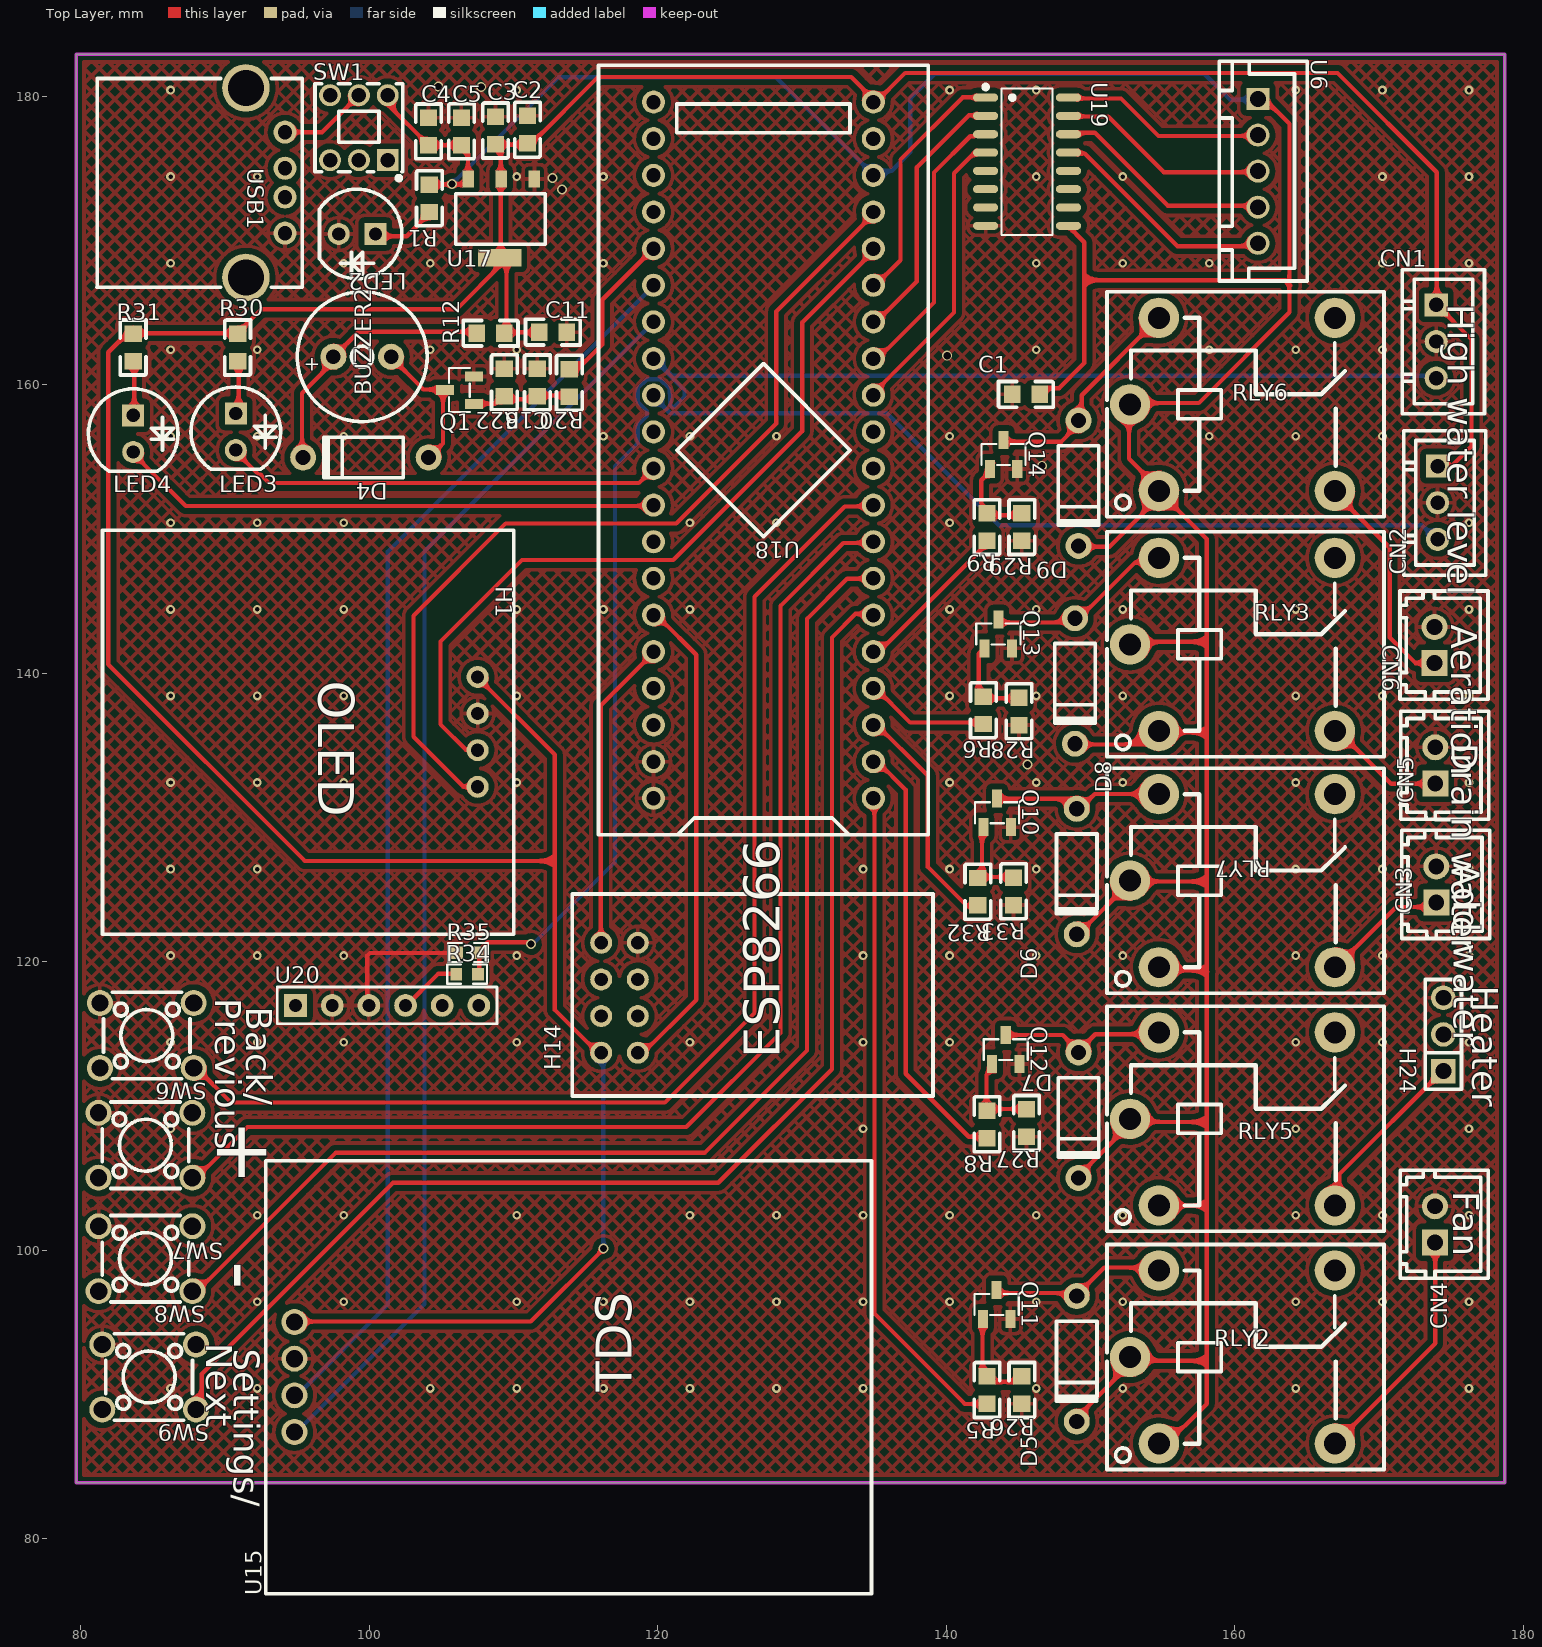
[diagram p0: Top Layer view]
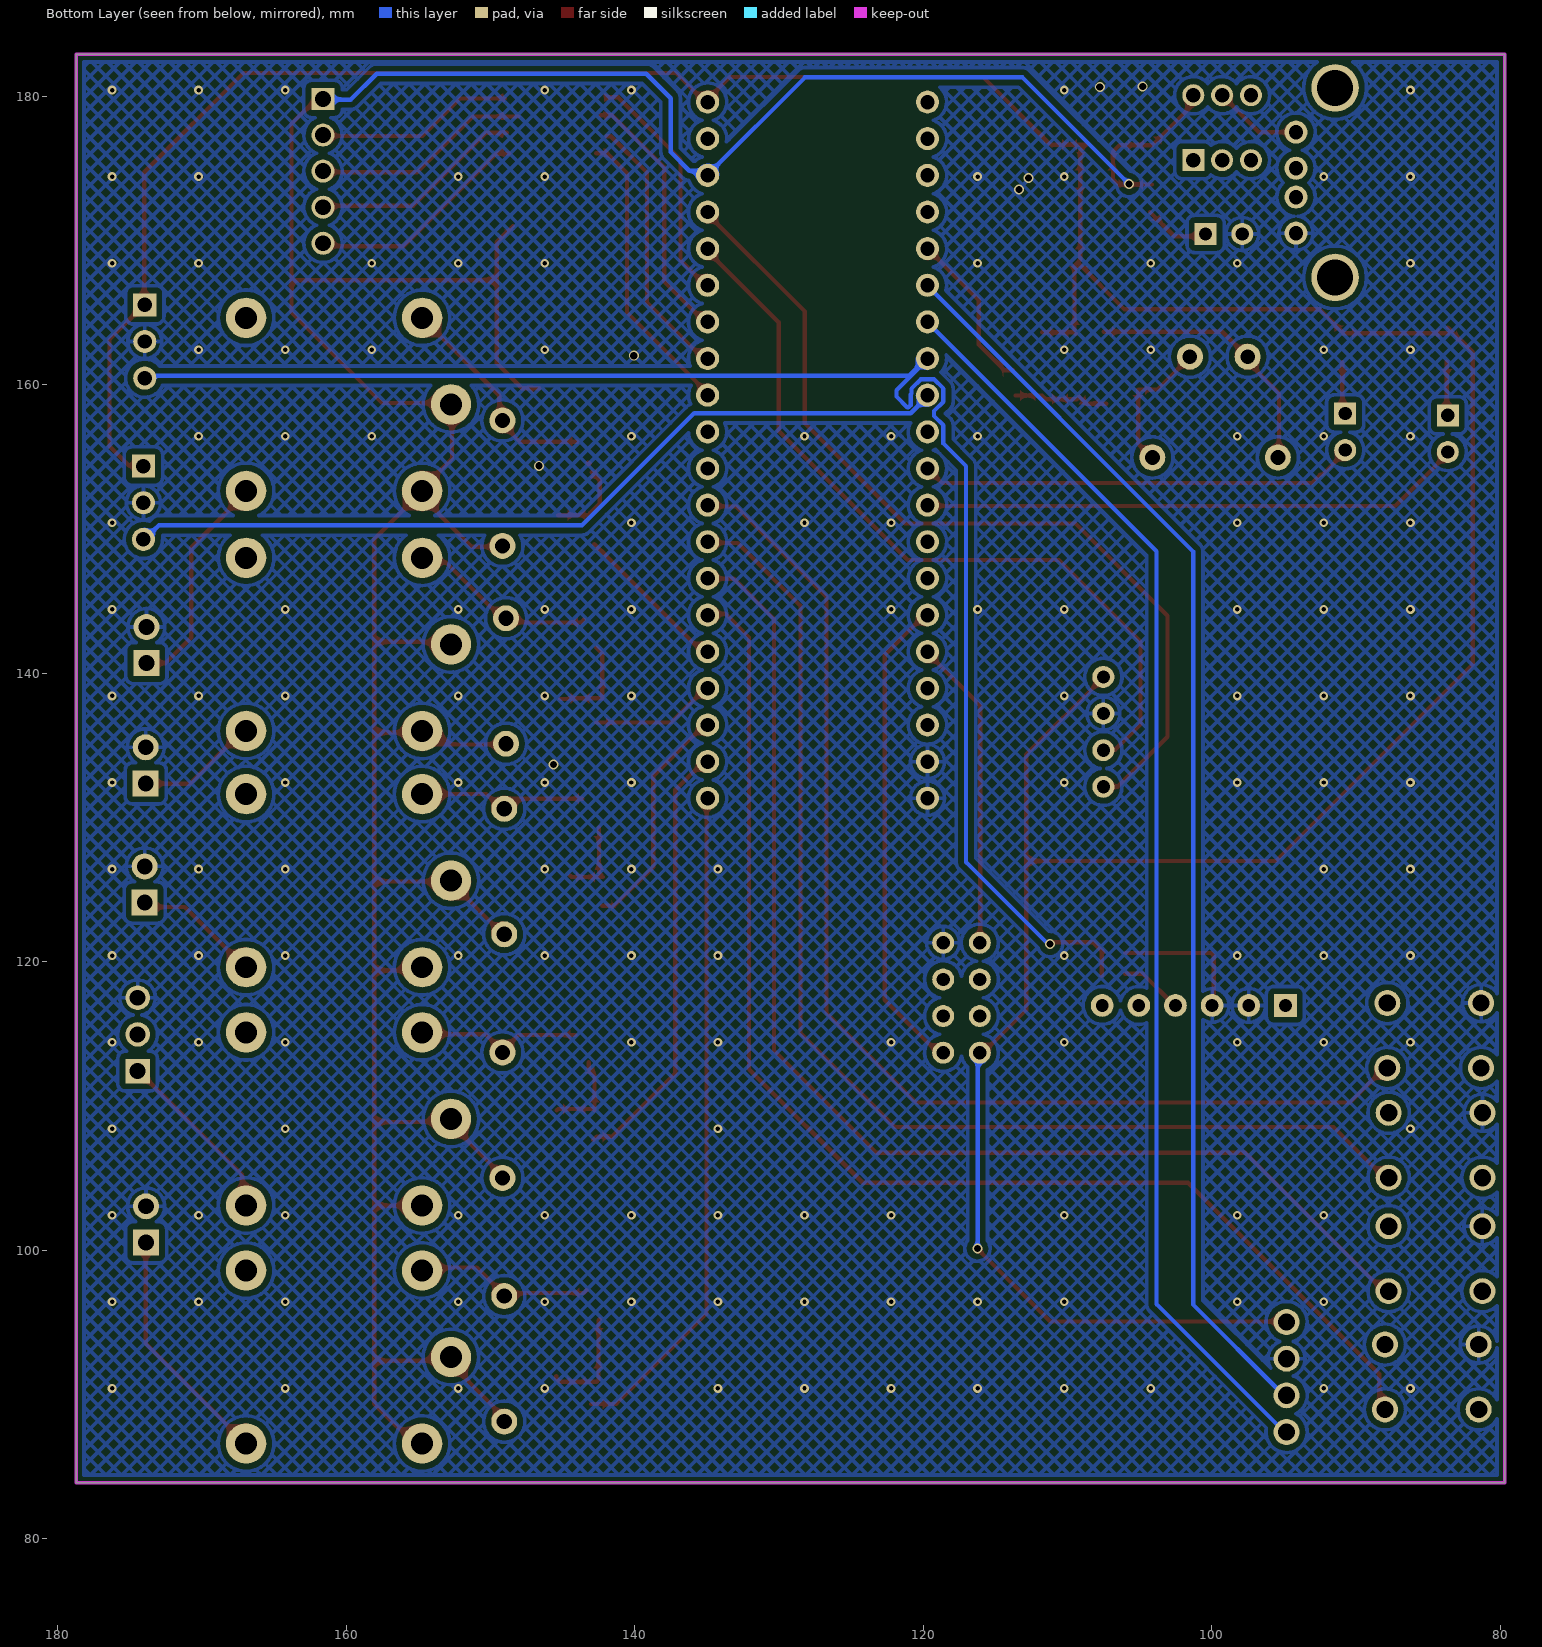
[diagram p1: Bottom Layer view, seen from below]
# Altium PCB MISC62619.pcbdoc
Units mm, origin at the board's own origin, x right, y up, seen from the top; angles counter-clockwise.
Board outline 99 x 99 mm, 2 copper layers (Top Layer, Bottom Layer), stack 1.58 mm thick; 67 components, 55 nets, 245 pads, 159 vias.

## Layer stack, top to bottom
Top Solder Mask Layer: solder mask 0.01, Dk 3.3
Top Layer: signal copper 0.035
Dielectric1: surface 1.51, FR4, Dk 4.5
Bottom Layer: signal copper 0.035
Bottom Solder Mask Layer: solder mask 0.01, Dk 3.3

## Board outline
79.696,182.894 79.696,83.894 178.696,83.894 178.696,182.894

## Design rules (kind name [scope] priority, off if disabled: settings)
BoardOutlineClearance copperThickness2oz_1 [All] p2 off: genericclearance=0.203 ignorepadtopadclearanceinfootprint=FALSE except(0: Arc-SplitContinuation Track-SplitContinuation SMDPad-SplitContinuation THPad-SplitContinuation Via-SplitContinuation Fill-SplitContinuation Region-SplitContinuation Poly-SplitContinuation Text-SplitContinuation Hole-SplitContinuation; 0.152: SMDPad-CutoutEdge THPad-CutoutEdge Via-CutoutEdge Fill-CutoutEdge Region-CutoutEdge Text-CutoutEdge Hole-CutoutEdge; 0.254: Poly-OutlineEdge Poly-CutoutEdge; 0.3: Arc-OutlineEdge Track-OutlineEdge SMDPad-OutlineEdge THPad-OutlineEdge Via-OutlineEdge Fill-OutlineEdge Region-OutlineEdge Text-OutlineEdge Hole-OutlineEdge Arc-CutoutEdge Track-CutoutEdge)
BoardOutlineClearance Plane_innerPlane_1 [All] p4 off: genericclearance=0.102 ignorepadtopadclearanceinfootprint=FALSE except(0: Arc-SplitContinuation Track-SplitContinuation SMDPad-SplitContinuation THPad-SplitContinuation Via-SplitContinuation Fill-SplitContinuation Region-SplitContinuation Poly-SplitContinuation Text-SplitContinuation Hole-SplitContinuation; 0.152: SMDPad-CutoutEdge THPad-CutoutEdge Via-CutoutEdge Fill-CutoutEdge Region-CutoutEdge Text-CutoutEdge Hole-CutoutEdge; 0.254: Poly-OutlineEdge Poly-CutoutEdge; 0.3: Arc-OutlineEdge Track-OutlineEdge SMDPad-OutlineEdge THPad-OutlineEdge Via-OutlineEdge Fill-OutlineEdge Region-OutlineEdge Text-OutlineEdge Hole-OutlineEdge Arc-CutoutEdge Track-CutoutEdge)
BoardOutlineClearance Copper_copperRegion_1 [All] p6 off: genericclearance=0.102 ignorepadtopadclearanceinfootprint=FALSE except(0: Arc-SplitContinuation Track-SplitContinuation SMDPad-SplitContinuation THPad-SplitContinuation Via-SplitContinuation Fill-SplitContinuation Region-SplitContinuation Poly-SplitContinuation Text-SplitContinuation Hole-SplitContinuation; 0.152: SMDPad-CutoutEdge THPad-CutoutEdge Via-CutoutEdge Fill-CutoutEdge Region-CutoutEdge Text-CutoutEdge Hole-CutoutEdge; 0.254: Poly-OutlineEdge Poly-CutoutEdge; 0.3: Arc-OutlineEdge Track-OutlineEdge SMDPad-OutlineEdge THPad-OutlineEdge Via-OutlineEdge Fill-OutlineEdge Region-OutlineEdge Text-OutlineEdge Hole-OutlineEdge Arc-CutoutEdge Track-CutoutEdge)
BoardOutlineClearance Copper_copperRegion1_1 [All] p8 off: genericclearance=0.102 ignorepadtopadclearanceinfootprint=FALSE except(0: Arc-SplitContinuation Track-SplitContinuation SMDPad-SplitContinuation THPad-SplitContinuation Via-SplitContinuation Fill-SplitContinuation Region-SplitContinuation Poly-SplitContinuation Text-SplitContinuation Hole-SplitContinuation; 0.152: SMDPad-CutoutEdge THPad-CutoutEdge Via-CutoutEdge Fill-CutoutEdge Region-CutoutEdge Text-CutoutEdge Hole-CutoutEdge; 0.3: Arc-OutlineEdge Track-OutlineEdge SMDPad-OutlineEdge THPad-OutlineEdge Via-OutlineEdge Fill-OutlineEdge Region-OutlineEdge Text-OutlineEdge Hole-OutlineEdge Arc-CutoutEdge Track-CutoutEdge; 0.4: Poly-OutlineEdge Poly-CutoutEdge)
BoardOutlineClearance copperThickness1oz_1 [All] p10: genericclearance=0.102 ignorepadtopadclearanceinfootprint=FALSE except(0: Arc-SplitContinuation Track-SplitContinuation SMDPad-SplitContinuation THPad-SplitContinuation Via-SplitContinuation Fill-SplitContinuation Region-SplitContinuation Poly-SplitContinuation Text-SplitContinuation Hole-SplitContinuation; 0.152: SMDPad-CutoutEdge THPad-CutoutEdge Via-CutoutEdge Fill-CutoutEdge Region-CutoutEdge Text-CutoutEdge Hole-CutoutEdge; 0.254: Poly-OutlineEdge Poly-CutoutEdge; 0.3: Arc-OutlineEdge Track-OutlineEdge SMDPad-OutlineEdge THPad-OutlineEdge Via-OutlineEdge Fill-OutlineEdge Region-OutlineEdge Text-OutlineEdge Hole-OutlineEdge Arc-CutoutEdge Track-CutoutEdge)
Clearance copperThickness2oz [All] p1 off: gap=0.203 ignorepadtopadclearanceinfootprint=FALSE except(0.152: SMDPad-Track SMDPad-SMDPad THPad-Track SMDPad-THPad THPad-THPad Track-Via SMDPad-Via THPad-Via Via-Via Fill-Track Region-Track Fill-SMDPad Region-SMDPad Fill-THPad Region-THPad Fill-Via Region-Via Fill-Fill Fill-Region Region-Region Arc-Track Arc-SMDPad Arc-THPad Arc-Via Fill-Arc Region-Arc Arc-Arc Text-Track SMDPad-Text Text-THPad Text-Via Fill-Text Region-Text Arc-Text Text-Text Hole-Track Hole-SMDPad Hole-THPad Hole-Via Fill-Hole Region-Hole Hole-Arc Hole-Text; 0.254: Poly-Track Poly-SMDPad Poly-THPad Poly-Via Poly-Fill Poly-Region Poly-Poly Poly-Arc Poly-Text Poly-Hole)
Clearance Plane_innerPlane [All] p3 off: gap=0.102 ignorepadtopadclearanceinfootprint=FALSE except(0.152: SMDPad-Track SMDPad-SMDPad THPad-Track SMDPad-THPad THPad-THPad Track-Via SMDPad-Via THPad-Via Via-Via Fill-Track Region-Track Fill-SMDPad Region-SMDPad Fill-THPad Region-THPad Fill-Via Region-Via Fill-Fill Fill-Region Region-Region Arc-Track Arc-SMDPad Arc-THPad Arc-Via Fill-Arc Region-Arc Arc-Arc Text-Track SMDPad-Text Text-THPad Text-Via Fill-Text Region-Text Arc-Text Text-Text Hole-Track Hole-SMDPad Hole-THPad Hole-Via Fill-Hole Region-Hole Hole-Arc Hole-Text; 0.254: Poly-Track Poly-SMDPad Poly-THPad Poly-Via Poly-Fill Poly-Region Poly-Poly Poly-Arc Poly-Text Poly-Hole)
Clearance Copper_copperRegion [All] p5 off: gap=0.102 ignorepadtopadclearanceinfootprint=FALSE except(0.152: SMDPad-Track SMDPad-SMDPad THPad-Track SMDPad-THPad THPad-THPad Track-Via SMDPad-Via THPad-Via Via-Via Fill-Track Region-Track Fill-SMDPad Region-SMDPad Fill-THPad Region-THPad Fill-Via Region-Via Fill-Fill Fill-Region Region-Region Arc-Track Arc-SMDPad Arc-THPad Arc-Via Fill-Arc Region-Arc Arc-Arc Text-Track SMDPad-Text Text-THPad Text-Via Fill-Text Region-Text Arc-Text Text-Text Hole-Track Hole-SMDPad Hole-THPad Hole-Via Fill-Hole Region-Hole Hole-Arc Hole-Text; 0.254: Poly-Track Poly-SMDPad Poly-THPad Poly-Via Poly-Fill Poly-Region Poly-Poly Poly-Arc Poly-Text Poly-Hole)
Clearance Copper_copperRegion1 [All] p7 off: gap=0.102 ignorepadtopadclearanceinfootprint=FALSE except(0.152: SMDPad-Track SMDPad-SMDPad THPad-Track SMDPad-THPad THPad-THPad Track-Via SMDPad-Via THPad-Via Via-Via Fill-Track Region-Track Fill-SMDPad Region-SMDPad Fill-THPad Region-THPad Fill-Via Region-Via Fill-Fill Fill-Region Region-Region Arc-Track Arc-SMDPad Arc-THPad Arc-Via Fill-Arc Region-Arc Arc-Arc Text-Track SMDPad-Text Text-THPad Text-Via Fill-Text Region-Text Arc-Text Text-Text Hole-Track Hole-SMDPad Hole-THPad Hole-Via Fill-Hole Region-Hole Hole-Arc Hole-Text; 0.4: Poly-Track Poly-SMDPad Poly-THPad Poly-Via Poly-Fill Poly-Region Poly-Poly Poly-Arc Poly-Text Poly-Hole)
Clearance copperThickness1oz [All] p9: gap=0.102 ignorepadtopadclearanceinfootprint=FALSE except(0.152: SMDPad-Track SMDPad-SMDPad THPad-Track SMDPad-THPad THPad-THPad Track-Via SMDPad-Via THPad-Via Via-Via Fill-Track Region-Track Fill-SMDPad Region-SMDPad Fill-THPad Region-THPad Fill-Via Region-Via Fill-Fill Fill-Region Region-Region Arc-Track Arc-SMDPad Arc-THPad Arc-Via Fill-Arc Region-Arc Arc-Arc Text-Track SMDPad-Text Text-THPad Text-Via Fill-Text Region-Text Arc-Text Text-Text Hole-Track Hole-SMDPad Hole-THPad Hole-Via Fill-Hole Region-Hole Hole-Arc Hole-Text; 0.254: Poly-Track Poly-SMDPad Poly-THPad Poly-Via Poly-Fill Poly-Region Poly-Poly Poly-Arc Poly-Text Poly-Hole)
DiffPairsRouting differentialPair [All] p1: maxlimit=0.152 minlimit=0.152 mostfreqgap=0.152 toplayer_minwidth=0.127 toplayer_prefwidth=0.254 toplayer_maxwidth=2.54 toplayer_mingap=0.152 toplayer_prefgap=0.152 toplayer_maxgap=0.152 bottomlayer_minwidth=0.127 bottomlayer_prefwidth=0.254 bottomlayer_maxwidth=2.54 bottomlayer_mingap=0.152 bottomlayer_prefgap=0.152 bottomlayer_maxgap=0.152 maxuncoupledlength=0.254
HoleToHoleClearance otherClearance [All] p1: gap=0.3 allowstackedmicrovias=TRUE
Length netLength [All] p1: minlimit=0 maxlimit=0
PasteMaskExpansion pasteMaskExpansion [All] p1: expansion=0
PlaneConnect innerPlane [All] p1: planeconnectstyle=Relief reliefexpansion=0.508 reliefentries=4 reliefconductorwidth=0.254 reliefairgap=0.254
PolygonConnect copperRegion1 [All] p1 off: connectstyle=Relief reliefconductorwidth=0.254 reliefentries=4 polygonreliefangle="90 Angle" airgapwidth=0.254 via.connectstyle=Relief via.reliefconductorwidth=0.254 via.reliefentries=4 via.polygonreliefangle="90 Angle" via.airgapwidth=0.254
PolygonConnect copperRegion [All] p2: connectstyle=Relief reliefconductorwidth=0.254 reliefentries=4 polygonreliefangle="90 Angle" airgapwidth=0.254 via.connectstyle=Relief via.reliefconductorwidth=0.254 via.reliefentries=4 via.polygonreliefangle="90 Angle" via.airgapwidth=0.254
RoutingVias viaSize [All] p1: holewidth=0.305 width=0.61 viastyle="Through Hole" minholewidth=0.3 minwidth=0.5 maxholewidth=6.3 maxwidth=10
SolderMaskExpansion solderMaskExpansion [IsVia] p1: expansion=-25.4 istentingtop=TRUE
SolderMaskExpansion solderMaskExpansion [All] p2: expansion=0.051 istentingtop=FALSE
Width copperThickness2oz_2 [All] p1 off: maxlimit=2.54 minlimit=0.203 preferedwidth=0.254
Width copperThickness1oz_2 [All] p2: maxlimit=2.54 minlimit=0.127 preferedwidth=0.254

## Components (designator, comment, footprint, x,y, rotation, side; value= is the part's Value field where it differs from the comment)
BUZZER2 "2.7kHz" BUZ-TH_BD9.0-P4.00-D0.6-FD 99.508,161.939 r0 top
C1 "100nF" c0805 145.515,159.327 r0 top
C2 "0.1u" c0805 110.961,177.682 r270 top
C3 "10u" c0805 108.746,177.621 r270 top
C4 "10u" c0805 104.103,177.555 r270 top
C5 "0.1u" c0805 106.384,177.56 r270 top
C11 "104/0603" c0805 112.726,163.637 r180 top
C16 "104/0603" c0805 111.644,160.149 r270 top
CN1 "ZX-XH2.54-3PZZ" CONN-TH_3P-P2.54_2501S-3P 173.956,162.995 r270 top
CN2 "ZX-XH2.54-3PZZ" CONN-TH_3P-P2.54_2501S-3P 174.05,151.817 r270 top
CN3 "ZX-XH2.54-2PZZ" CONN-TH_2P-P2.50_HX25003-2A 173.961,125.357 r90 top
CN4 "ZX-XH2.54-2PZZ" CONN-TH_2P-P2.50_HX25003-2A 173.867,101.798 r90 top
CN5 "ZX-XH2.54-2PZZ" CONN-TH_2P-P2.50_HX25003-2A 173.891,133.615 r90 top
CN6 "ZX-XH2.54-2PZZ" CONN-TH_2P-P2.50_HX25003-2A 173.843,141.95 r90 top
D4 "1N4007" DO-41_BD2.4-L4.7-P8.70-D0.8-RD 99.762,154.954 r0 top
D5 "1N4007" DO-41_BD2.4-L4.7-P8.70-D0.8-RD 149.038,92.47 r90 top
D6 "1N4007" DO-41_BD2.4-L4.7-P8.70-D0.8-RD 149.038,126.252 r90 top
D7 "1N4007" DO-41_BD2.4-L4.7-P8.70-D0.8-RD 149.165,109.361 r90 top
D8 "1N4007" DO-41_BD2.4-L4.7-P8.70-D0.8-RD 148.911,139.46 r90 top
D9 "1N4007" DO-41_BD2.4-L4.7-P8.70-D0.8-RD 149.165,153.176 r90 top
H1 "OLED" oled 107.509,135.904 r270 top
H14 "PZ254V-12-8P" esp8266 116.073,117.691 r90 top
H24 "Heater" HDR-TH_3P-P2.54-V-M 174.454,114.961 r90 top
LED2 "L-7113SGC" LED-TH_BD5.9-P2.54-FD 99.15,170.448 r180 top
LED3 "L-7113SGC" LED-TH_BD5.9-P2.54-FD 90.745,156.732 r270 top
LED4 "L-7113SGC" LED-TH_BD5.9-P2.54-FD 83.633,156.605 r270 top
Q1 "SS8050/SOT23-3" SOT-23-3_L2.9-W1.3-P1.90-LS2.4-BR 106.242,159.623 r0 top
Q10 "SS8050/SOT23-3" SOT-23-3_L2.9-W1.3-P1.90-LS2.4-BR 143.517,130.324 r270 top
Q11 "SS8050/SOT23-3" SOT-23-3_L2.9-W1.3-P1.90-LS2.4-BR 143.486,96.231 r270 top
Q12 "SS8050/SOT23-3" SOT-23-3_L2.9-W1.3-P1.90-LS2.4-BR 144.116,113.905 r270 top
Q13 "SS8050/SOT23-3" SOT-23-3_L2.9-W1.3-P1.90-LS2.4-BR 143.603,142.722 r270 top
Q14 "SS8050/SOT23-3" SOT-23-3_L2.9-W1.3-P1.90-LS2.4-BR 143.965,155.161 r270 top
R1 "" c0805 104.164,172.922 r270 top
R5 "" c0805 142.815,90.311 r90 top
R6 "" c0805 142.561,137.428 r90 top
R8 "" c0805 142.815,108.726 r90 top
R9 "" c0805 142.815,150.128 r90 top
R12 "220" c0805 108.406,163.565 r180 top
R20 "1K/0603" c0805 113.862,160.126 r270 top
R22 "10K/0603" c0805 109.361,160.162 r270 top
R26 "10K/0603" c0805 145.228,90.311 r90 top
R27 "10K/0603" c0805 145.55,108.827 r90 top
R28 "10K/0603" c0805 145.04,137.357 r90 top
R29 "10K/0603" c0805 145.228,150.128 r90 top
R30 "" c0805 90.872,162.574 r90 top
R31 "" c0805 83.633,162.574 r90 top
R32 "" c0805 142.18,124.855 r90 top
R33 "10K/0603" c0805 144.654,124.879 r90 top
R34 "2.2K" R0603 106.782,119.138 r0 top
R35 "3.3K" R0603 106.834,120.636 r0 top
RLY2 "SRD-05VDC-SL-C" RELAY-TH_SRD-XXVDC-XL-C 159.833,92.597 r0 top
RLY3 "SRD-05VDC-SL-C" RELAY-TH_SRD-XXVDC-XL-C 159.833,142 r0 top
RLY5 "SRD-05VDC-SL-C" RELAY-TH_SRD-XXVDC-XL-C 159.833,109.107 r0 top
RLY6 "SRD-05VDC-SL-C" RELAY-TH_SRD-XXVDC-XL-C 159.833,158.637 r0 top
RLY7 "SRD-05VDC-SL-C" RELAY-TH_SRD-XXVDC-XL-C 159.833,125.617 r0 top
SW1 "5.8 ZSGT" SW-TH_5.8ZSGT 99.277,177.814 r0 top
SW6 "TS665CJ" SW-TH_4P-L6.0-W6.0-P4.50-LS6.5 84.575,114.883 r180 top
SW7 "TS665CJ" SW-TH_4P-L6.0-W6.0-P4.50-LS6.5 84.48,107.28 r180 top
SW8 "TS665CJ" SW-TH_4P-L6.0-W6.0-P4.50-LS6.5 84.484,99.414 r180 top
SW9 "TS665CJ" SW-TH_4P-L6.0-W6.0-P4.50-LS6.5 84.738,91.217 r180 top
U6 "ZX-XH2.54-5PZZ" CONN-TH_5P-P2.50_ZX-XH2.54-5PZZ 161.602,174.802 r270 top
U15 "" TDS模块 94.809,91.2 r90 top
U17 "AMS1117-3.3" sot-223 111.446,174.258 r270 top
U18 "LCKFB-DKX-STM32F103C8T6" CONN-TH_L53.3-W22.9_STM32F103C8T6-CARD 127.321,155.462 r90 top
U19 "ULN2003A" SOP-16_L10.0-W3.9-P1.27-LS6.0-BL 145.594,175.457 r270 top
U20 "" HDR-M-2.54_1X6 101.239,116.969 r0 top
USB1 "USB-231-ARY" USB-A-TH_USB-231-ARY 92.8,174.004 r270 top

## Footprints (in the part's own frame and the unit in brackets; to place one, negate y for a bottom-side part, rotate by r counter-clockwise, add the part's x,y. Pads: shape width x height; smd on the part's side, far side on the other; paste and mask are expansions set on the pad)
BUZ-TH_BD9.0-P4.00-D0.6-FD [mm]
  round 1.8 hole 1: 1(-2,0) 2(2,0)
  silkscreen extent -4.5,-4.5 4.5,4.5
c0805 [mm]
  rect 1.14x1.2 smd: 1(-0.95,0) 2(0.95,0)
  silkscreen extent -1.91,-0.89 1.91,0.89
CONN-TH_2P-P2.50_HX25003-2A [mm]
  rect 1.8x1.8 hole 1.1 paste+0 mask+0.05: 1(-1.25,0)
  round 1.8 hole 1.1 paste+0 mask+0.05: 2(1.25,0)
  silkscreen extent -3.75,-3.7 3.75,2.41
CONN-TH_3P-P2.54_2501S-3P [mm]
  rect 1.6x1.6 hole 1: 1(-2.54,0)
  round 1.6 hole 1: 2(0,0) 3(2.54,0)
  silkscreen extent -4.98,-2.35 5.02,3.35
CONN-TH_5P-P2.50_ZX-XH2.54-5PZZ [mm]
  rect 1.524x1.6 hole 1.1: 1(-5,0)
  round 1.6 hole 1.1: 2(-2.5,0) 3(0,0) 4(2.5,0) 5(5,0)
  silkscreen extent -7.62,-2.68 7.62,3.42
CONN-TH_L53.3-W22.9_STM32F103C8T6-CARD [mm]
  round 1.6 hole 1: 1(-24.13,-7.62) 2(-21.59,-7.62) 3(-19.05,-7.62) 4(-16.51,-7.62) 5(-13.97,-7.62) 6(-11.43,-7.62) 7(-8.89,-7.62) 8(-6.35,-7.62) 9(-3.81,-7.62) 10(-1.27,-7.62) 11(1.27,-7.62) 12(3.81,-7.62) 13(6.35,-7.62) 14(8.89,-7.62) 15(11.43,-7.62) 16(13.97,-7.62) 17(16.51,-7.62) 18(19.05,-7.62) 19(21.59,-7.62) 20(24.13,-7.62) 21(24.13,7.62) 22(21.59,7.62) 23(19.05,7.62) 24(16.51,7.62) 25(13.97,7.62) 26(11.43,7.62) 27(8.89,7.62) 28(6.35,7.62) 29(3.81,7.62) 30(1.27,7.62) 31(-1.27,7.62) 32(-3.81,7.62) 33(-6.35,7.62) 34(-8.89,7.62) 35(-11.43,7.62) 36(-13.97,7.62) 37(-16.51,7.62) 38(-19.05,7.62) 39(-21.59,7.62) 40(-24.13,7.62)
  silkscreen extent -26.67,-11.43 26.67,11.43
DO-41_BD2.4-L4.7-P8.70-D0.8-RD [mm]
  round 1.8 hole 1.05: 1(-4.35,0) 2(4.35,0)
  silkscreen extent -2.92,-1.4 2.6,1.4
esp8266 [mil]
  round 60 hole 36: 1(-157.48,0) 2(-157.48,-100) 3(-57.48,0) 4(-57.48,-100) 5(42.52,0) 6(42.52,-100) 7(142.52,0) 8(142.52,-100)
  silkscreen extent -276,-906 276,79
HDR-M-2.54_1X6 [mil]
  rect 62x62 hole 35: 1(-250,0)
  round 62 hole 35: 2(-150,0) 3(-50,0) 4(50,0) 5(150,0) 6(250,0)
  silkscreen extent -300,-50 300,50
HDR-TH_3P-P2.54-V-M [mm]
  rect 1.7x1.7 hole 1.1: 1(-2.54,0)
  round 1.7 hole 1.1: 2(0,0) 3(2.54,0)
  silkscreen extent -3.81,-1.25 3.81,1.25
LED-TH_BD5.9-P2.54-FD [mil]
  rect 60x60 hole 36: 1(-50,0)
  round 60 hole 36: 2(50,0)
  silkscreen extent -122,-122 102,122
oled [mil]
  round 60 hole 36: 1(148.82,0) 2(48.82,0) 3(-51.18,0) 4(-151.18,0)
  silkscreen extent -551,-1024 551,98
R0603 [mm]
  rect 0.806x0.864 smd paste-100 mask+0.051: 1(-0.753,0) 2(0.753,0)
  silkscreen extent -1.39,-0.66 1.39,0.66
RELAY-TH_SRD-XXVDC-XL-C [mil]
  round 110 hole 60: 1(-200.79,-236.22) 2(279.52,-236.2) 3(279.53,236.2) 4(-200.79,236.22) 5(-279.53,0)
  silkscreen extent -342,-307 413,307
SOP-16_L10.0-W3.9-P1.27-LS6.0-BL [mm]
  oval 0.56x1.745 smd: 1(-4.445,-2.872) 2(-3.175,-2.872) 3(-1.905,-2.872) 4(-0.635,-2.872) 5(0.635,-2.872) 6(1.905,-2.872) 7(3.175,-2.872) 8(4.445,-2.872) 9(4.445,2.872) 10(3.175,2.872) 11(1.905,2.872) 12(0.635,2.872) 13(-0.635,2.872) 14(-1.905,2.872) 15(-3.175,2.872) 16(-4.445,2.872)
  silkscreen extent -5.33,-3.02 5.08,1.77
SOT-23-3_L2.9-W1.3-P1.90-LS2.4-BR [mm]
  rect 1.25x0.7 smd: 1(1,-0.95) 2(1,0.95) 3(-1,0)
  silkscreen extent -0.73,-1.53 0.73,1.53
sot-223 [mm]
  rect 1.2x0.8 smd: 1(0,0) 2(0,-2.3) 3(0,-4.6)
  rect 1.2x3 smd: 4(5.461,-2.413)
  silkscreen extent 1.02,-5.46 4.52,0.74
SW-TH_4P-L6.0-W6.0-P4.50-LS6.5 [mm]
  round 1.8 hole 1.2: 1(-3.25,2.25) 2(3.25,2.25) 3(-3.25,-2.25) 4(3.25,-2.25)
  silkscreen extent -3,-3 3,3
SW-TH_5.8ZSGT [mm]
  rect 1.524x1.524 hole 1: 1(2,-2.25)
  round 1.524 hole 1: 2(0,-2.25) 3(-2,-2.25) 4(2,2.25) 5(0,2.25) 6(-2,2.25)
  silkscreen extent -3.05,-3.64 3.05,3.05
TDS模块 [mm]
  round 1.8 hole 1.2: 1(-3.8,0) 2(-1.26,0) 3(1.28,0) 4(3.82,0)
  silkscreen extent -15,-40 15,2
USB-A-TH_USB-231-ARY [mm]
  round 1.6 hole 1: 1(-3.5,1.355) 2(-1,1.355) 3(1,1.355) 4(3.5,1.355)
  round 3.3 hole 2.5: 5(-6.57,-1.355) 6(6.57,-1.355)
  silkscreen extent -7.23,-11.68 7.24,2.54

## Via types
v1: diameter 0.61, hole 0.305, Top Layer to Bottom Layer, 149 vias
v2: diameter 0.7, hole 0.5, Top Layer to Bottom Layer, 10 vias

## Nets (pads, with @x,y where several pads share a name; then routed paths per layer and width w, separated by ;. In a path a pad name is that pad's centre, name@x,y a point inside that pad or via, vN(x,y) a via of type N, cw(c..) or ccw(c..) an arc to the next point about the centre after c; other vN are vias at no path point)
3.3V: C2.2 C3.2 C11.2 CN1.1 CN2.1 H1.4 H14.1 R12.1 R30.2 R31.2 U15.4 U17.2 U17.4 U18.20 | length 265.4
  Top Layer w0.3: R31.2@83.574,163.591 83.596,163.569 R30.2@90.895,163.569 ; R31.2@83.626,163.968 81.905,162.247 81.905,140.613 95.532,126.986 112.846,126.986 ; R30.2@90.842,163.571 92.493,165.222 106.038,165.222 U17.4@109.275,168.459 ; U15.4@94.801,95.059 111.192,95.059 v2@116.295,100.162 ; H1.4@107.612,139.592 112.863,134.342 112.863,116.659 H14.1@115.995,113.527 ; U17.4@109.14,168.672 109.111,168.701 109.111,176.219 108.689,176.642 111.005,176.642 C2.2@111.064,176.584 ; U17.4@109.189,168.564 109.514,168.24 R12.1@109.514,163.769 ; R12.1@109.428,163.536 109.516,163.624 C11.2@111.745,163.624 ; C2.2@111.225,176.691 115.858,181.324 133.407,181.324 U18.20@135.046,179.685 ; U18.20@134.985,179.447 137.139,181.601 167.117,181.601 173.997,174.721 CN1.1@173.997,165.548 ; CN1.1@173.807,165.737 CN1.1@173.997,165.548 ; CN1.1@173.997,165.535 CN1.1@173.997,165.548 ; CN2.1@174.018,154.393 175.072,154.393 176.406,155.728 176.406,163.138 CN1.1@173.997,165.548
  Bottom Layer w0.3: H14.1@116.224,113.697 116.224,100.132 v2(116.235,100.12)
5V: C1.2 C4.2 C5.2 D5.1 D6.1 D7.1 D8.1 D9.1 R1.1 RLY2.1 RLY2.5 RLY3.1 RLY3.5 RLY5.1 RLY5.5 RLY6.1 RLY6.5 RLY7.1 RLY7.5 SW1.4 U6.1 U17.3 U18.18 U19.9 | length 273.1
  Top Layer w0.3: SW1.4 101.277,179.431 C4.2 106.379,176.605 C5.2 106.846,176.148 U17.3 106.46,173.872 R1.1 ; C1.2@146.591,159.764 147.826,159.764 149.565,161.502 149.565,167.244 ; U19.9@148.427,171 149.554,169.873 ; D6.1@148.84,122.055 149.292,122.055 RLY7.5@152.711,125.473 ; D5.1@149.022,88.387 RLY2.5@152.971,92.337 ; D7.1@149.128,105.128 RLY5.5@152.89,108.89 ; D8.1@149.145,135.057 RLY3.1@153.931,135.057 ; D9.1@149.178,148.76 151.308,148.76 154.882,152.333 RLY6.1@154.882,152.47 ; 149.565,169.873 149.565,167.244 ; RLY6.5@152.664,158.731 157.503,158.731 163.789,165.018 163.789,166.942 ; RLY6.5@152.665,158.638 152.665,154.868 RLY6.1@154.96,152.574 ; RLY3.5@152.7,142.178 158.013,142.178 158.041,142.149 ; RLY2.5@152.705,92.337 RLY2.5@152.971,92.337 ; RLY7.5@152.804,125.567 158.018,125.567 ; RLY5.5@152.921,108.921 RLY5.5@152.89,108.89 ; RLY6.1@154.751,152.601 RLY6.1@154.882,152.47 ; RLY3.1@154.753,135.885 158.041,135.885 158.052,135.895 ; RLY5.1@154.8,103.089 157.984,103.089 157.994,103.099 ; RLY7.1@154.81,119.39 158.026,119.39 158.052,119.363 ; RLY2.1@154.953,86.252 158.052,89.352 158.052,108.89 ; 158.044,92.337 RLY2.5@153.096,92.337 ; 158.072,108.9 158.062,108.89 158.052,108.89 ; 158.072,135.916 158.052,135.895 ; 158.104,119.312 158.052,119.363 ; U6.1@161.928,179.944 163.789,178.083 163.789,166.942 ; 163.858,166.873 163.789,166.942 ; 149.565,167.244 163.487,167.244 163.789,166.942 ; RLY5.5@152.89,108.89 158.052,108.89 ; RLY2.5@152.971,92.337 RLY2.5@153.096,92.337 ; RLY2.5@152.971,92.337 152.986,92.352 RLY2.5@153.096,92.337 ; RLY6.1@154.882,152.47 158.052,149.3 158.052,135.895 ; 158.052,108.89 158.052,119.363 ; 158.052,119.363 158.052,135.895
  Bottom Layer w0.3: v2(105.729,173.914) 113.117,181.302 128.201,181.302 U18.18@134.913,174.59 ; U18.18@134.794,174.584 U18.18@134.908,174.469 ; U18.18@134.95,174.531 135.25,174.831 136.207,174.831 137.499,176.124 137.499,179.859 139.196,181.556 157.88,181.556 159.675,179.761 U6.1@161.735,179.761
$1N861: U6.5 U19.13 | length 15.6
  Top Layer w0.3: U19.13@148.694,176.028 149.599,176.028 156.026,169.6 U6.5@161.616,169.6
$1N862: U6.4 U19.14 | length 14.7
  Top Layer w0.3: U19.14@148.872,177.461 150.295,177.461 155.343,172.413 U6.4@161.448,172.413
$1N863: U6.3 U19.15 | length 15.2
  Top Layer w0.3: U19.15@148.066,178.586 151.219,178.586 155.071,174.734 U6.3@161.677,174.734
$1N864: U6.2 U19.16 | length 13.9
  Top Layer w0.3: U19.16@149.003,179.834 149.006,179.837 152.102,179.837 154.704,177.235 161.79,177.235 U6.2@161.794,177.239
$1N1483: D5.2 Q11.3 RLY2.4 | length 12.5
  Top Layer w0.3: Q11.3@143.321,97.236 143.517,97.04 149.179,97.04 150.95,98.81 154.509,98.81 RLY2.4@154.873,98.446
$1N1484: CN4.1 RLY2.2 | length 16.6
  Top Layer w0.3: RLY2.2@167.061,86.716 173.888,93.543 CN4.1@173.888,100.51
$1N1737: D8.2 Q13.3 RLY3.4 | length 13.5
  Top Layer w0.3: Q13.3@143.518,143.714 143.716,143.516 D8.2@148.917,143.516 ; D8.2@149.188,143.516 D8.2@148.917,143.516 ; RLY3.4@154.947,147.678 153.079,147.678 D8.2@148.917,143.516
$1N1738: CN5.1 RLY3.2 | length 8.2
  Top Layer w0.3: RLY3.2@167.271,135.901 170.83,132.342 CN5.1@174.038,132.342
$1N2245: D7.2 Q12.3 RLY5.4 | length 11.5
  Top Layer w0.3: Q12.3@144.102,114.918 148.062,114.918 D7.2@149.165,113.814 ; D7.2@149.184,113.796 D7.2@149.165,113.814 ; RLY5.4@154.685,114.974 150.325,114.974 D7.2@149.165,113.814
$1N2246: H24.1 RLY5.2 | length 12.8
  Top Layer w0.3: RLY5.2@167.224,102.864 167.224,105.251 H24.1@174.553,112.58
$1N2555: D9.2 Q14.3 RLY6.4 | length 15.1
  Top Layer w0.3: Q14.3@143.968,156.055 147.98,156.055 D9.2@149.358,157.432 ; D9.2@149.385,157.305 149.385,159.272 154.47,164.357 RLY6.4@154.485,164.342
$1N2556: CN6.1 RLY6.2 | length 15.6
  Top Layer w0.3: RLY6.2@166.996,152.437 170.736,148.697 170.736,142.48 172.516,140.701 CN6.1@174.061,140.701
$1N5721: LED2.1 R1.2 | length 4.5
  Top Layer w0.3: LED2.1@100.442,170.289 102.599,170.289 R1.2@104.274,171.965
$1N6173: C16.2 Q1.1 R20.2 R22.2 | length 6.7
  Top Layer w0.3: Q1.1@107.309,158.681 108.707,158.681 109.188,159.162 109.363,158.987 111.505,158.987 111.767,159.25 R20.2@113.603,159.25
$1N6175: BUZZER2.2 D4.2 Q1.3 | length 9.9
  Top Layer w0.3: BUZZER2.2@101.342,162.069 103.746,159.665 105.101,159.665 105.101,155.928 D4.2@104.074,154.901
$1N6178: BUZZER2.1 D4.1 R12.2 | length 18.5
  Top Layer w0.3: D4.1@95.332,154.86 95.332,159.406 BUZZER2.1@97.627,161.701 ; BUZZER2.1@97.517,161.919 99.266,163.667 R12.2@107.483,163.667
$1N8726: Q11.1 R5.2 R26.2 | length 7.5
  Top Layer w0.3: Q11.1@142.429,95.211 142.501,95.139 142.501,91.008 142.632,90.876 145.186,90.876 145.432,91.122 R26.2@145.432,91.278
$1N8768: Q12.1 R8.2 R27.2 | length 6
  Top Layer w0.3: R8.2@142.785,109.696 142.785,112.154 143.19,112.56 Q12.1@143.19,113.024 ; R8.2@142.981,109.794 145.309,109.794 R27.2@145.407,109.696
$1N8808: Q13.1 R6.2 R28.2 | length 6.6
  Top Layer w0.3: Q13.1@142.668,141.782 142.236,141.35 142.236,138.255 144.552,138.255 144.596,138.211 R28.2@145.157,138.211
$1N8848: Q14.1 R9.2 R29.2 | length 5.8
  Top Layer w0.3: Q14.1@142.965,153.929 142.415,153.38 142.415,151.773 R9.2@143.069,151.118 ; R9.2@143.069,150.953 145.294,150.953 R29.2@145.304,150.963 ; Q14.1@143.106,154.553 143.173,154.486 143.24,154.553 143.24,154.578 Q14.1@143.228,154.589
$1N8939: LED3.1 R30.1 | length 3.6
  Top Layer w0.3: LED3.1@90.742,158.018 90.939,158.215 R30.1@90.939,161.559
$1N8963: LED4.1 R31.1 | length 3.8
  Top Layer w0.3: LED4.1@83.64,157.821 83.705,157.887 R31.1@83.705,161.602
$1N9376: D6.2 Q10.3 RLY7.4 | length 12
  Top Layer w0.3: Q10.3@143.64,131.302 148.519,131.302 D6.2@149.158,130.663 ; D6.2@149.21,130.556 150.281,131.627 RLY7.4@154.936,131.627
$1N9377: CN3.1 RLY7.2 | length 8.9
  Top Layer w0.3: RLY7.2@166.967,119.582 171.181,123.796 CN3.1@174.155,123.796
$1N9379: Q10.1 R32.2 R33.2 | length 5.6
  Top Layer w0.3: R32.2@142.206,125.877 144.372,125.877 R33.2@144.466,125.971 ; R32.2@142.299,126.017 142.471,126.189 Q10.1@142.471,129.291
$1N14885: SW1.5 USB1.1 | length 6.2
  Top Layer w0.3: USB1.1@94.155,177.504 96.717,177.504 SW1.5
$1N31715: R34.1 U20.4 | length 4.4
  Top Layer w0.3: U20.4@102.558,116.949 104.767,119.158 R34.1@106,119.158
+5V: U20.1
ACC: SW7.1 U18.8 | length 83.1
  Top Layer w0.3: SW7.1@87.597,104.83 87.842,104.83 91.554,108.543 121.976,108.543 128.497,115.064 128.497,144.668 132.857,149.028 134.824,149.028 U18.8@134.977,149.181
ACC_WATER: R32.1 U18.3 | length 16.3
  Top Layer w0.3: U18.3@134.924,136.685 138.717,132.892 138.717,126.571 141.398,123.89 R32.1@142.245,123.89
AIR: R9.1 U18.5 | length 11
  Top Layer w0.3: U18.5@134.819,141.532 135.38,141.532 R9.1@142.791,148.942
BACK: SW6.1 U18.9 | length 82.3
  Top Layer w0.3: SW6.1@87.756,112.475 88.18,112.475 90.413,110.242 120.489,110.242 126.701,116.454 126.701,145.303 132.951,151.553 U18.9@135.093,151.553
BUZZER_CTRL: R20.1 U18.25 | length 11.1
  Top Layer w0.3: R20.1@113.775,161.002 114.368,161.002 116.147,162.782 116.147,165.888 U18.25@119.581,169.322
DEC: SW8.1 U18.7 | length 85.6
  Top Layer w0.3: SW8.1@87.469,96.555 97.664,106.75 123.241,106.75 130.337,113.846 130.337,143.765 133.12,146.548 U18.7@134.857,146.548
DEC_WATER: R6.1 U18.4 | length 8.7
  Top Layer w0.3: U18.4@134.994,139.074 137.488,136.58 R6.1@142.65,136.58
ES8266_TX: H14.7 U18.36 | length 21.6
  Top Layer w0.3: H14.7@116.047,121.343 116.047,137.762 U18.36@119.732,141.447
ESP8266_RX: H14.2 U18.35 | length 33.5
  Top Layer w0.3: H14.2@118.796,113.491 122.659,117.354 122.659,141.283 120.218,143.724 U18.35@119.586,143.724
FAN: R5.1 U18.1 | length 46.3
  Top Layer w0.3: U18.1@135.019,131.281 135.019,95.608 141.285,89.343 R5.1@143.005,89.343
FAN_LED: LED4.2 U18.32 | length 37.6
  Top Layer w0.3: LED4.2@83.659,155.199 87.273,151.585 U18.32@119.756,151.585
GND: C1.1 C2.1 C3.1 C4.1 C5.1 C11.1 C16.1 CN1.2 CN2.2 CN3.2 CN4.2 CN5.2 CN6.2 H1.3 H14.8 H24.3 LED2.2 Q1.2 Q10.2 Q11.2 Q12.2 Q13.2 Q14.2 R22.1 R26.1 R27.1 R28.1 R29.1 R33.1 R35.1 SW6.4 SW7.4 SW8.4 SW9.4 U15.3 U17.1 U18.39 U18.40 U19.8 U20.2 U20.3 USB1.4 | length 9.6
  Top Layer w0.3: U20.3@99.86,117.065 99.86,120.437 100.023,120.6 R35.1@106,120.6
  other v1: 86.225,90.424 92.225,90.424 104.225,90.424 110.225,90.424 116.225,90.424 122.225,90.424 128.225,90.424 134.225,90.424 146.225,90.424 152.225,90.424 164.225,90.424 176.225,90.424 92.225,96.424 98.225,96.424 110.225,96.424 116.225,96.424 122.225,96.424 128.225,96.424 134.225,96.424 140.225,96.424 146.225,96.424 152.225,96.424 164.225,96.424 170.225,96.424 176.225,96.424 92.225,102.424 98.225,102.424 110.225,102.424 122.225,102.424 128.225,102.424 134.225,102.424 140.225,102.424 146.225,102.424 152.225,102.424 164.225,102.424 170.225,102.424 176.225,102.424 86.225,108.424 134.225,108.424 164.225,108.424 176.225,108.424 86.225,114.424 92.225,114.424 98.225,114.424 110.225,114.424 122.225,114.424 134.225,114.424 140.225,114.424 164.225,114.424 170.225,114.424 176.225,114.424 86.225,120.424 92.225,120.424 98.225,120.424 110.225,120.424 134.225,120.424 140.225,120.424 146.225,120.424 152.225,120.424 164.225,120.424 170.225,120.424 176.225,120.424 86.225,126.424 92.225,126.424 134.225,126.424 140.225,126.424 146.225,126.424 164.225,126.424 170.225,126.424 176.225,126.424 86.225,132.424 92.225,132.424 98.225,132.424 110.225,132.424 140.225,132.424 146.225,132.424 152.225,132.424 164.225,132.424 176.225,132.424 86.225,138.424 92.225,138.424 98.225,138.424 110.225,138.424 140.225,138.424 146.225,138.424 152.225,138.424 164.225,138.424 170.225,138.424 176.225,138.424 86.225,144.424 92.225,144.424 98.225,144.424 110.225,144.424 116.225,144.424 122.225,144.424 140.225,144.424 146.225,144.424 152.225,144.424 164.225,144.424 176.225,144.424 86.225,150.424 92.225,150.424 98.225,150.424 122.225,150.424 128.225,150.424 140.225,150.424 176.225,150.424 86.225,156.424 92.225,156.424 98.225,156.424 116.225,156.424 122.225,156.424 128.225,156.424 140.225,156.424 158.225,156.424 164.225,156.424 170.225,156.424 86.225,162.424 92.225,162.424 104.225,162.424 110.225,162.424 146.225,162.424 158.225,162.424 164.225,162.424 170.225,162.424 86.225,168.424 98.225,168.424 104.225,168.424 116.225,168.424 146.225,168.424 152.225,168.424 158.225,168.424 170.225,168.424 176.225,168.424 86.225,174.424 92.225,174.424 110.225,174.424 116.225,174.424 146.225,174.424 152.225,174.424 170.225,174.424 176.225,174.424 86.225,180.424 110.225,180.424 140.225,180.424 146.225,180.424 164.225,180.424 170.225,180.424 176.225,180.424
  other v2: 145.624,133.677 146.635,154.375 140.057,162.011 113.366,173.534 112.689,174.319 107.754,180.642 104.782,180.673
HEAT: R8.1 U18.2 | length 30
  Top Layer w0.3: U18.2@135.259,133.839 137.185,131.914 137.185,112.24 141.552,107.873 142.629,107.873 R8.1@142.863,107.639
HEAT_LED: LED3.2 U18.31 | length 30.3
  Top Layer w0.3: LED3.2@90.602,155.491 92.322,153.77 92.463,153.77 93.048,153.185 118.686,153.185 U18.31@119.576,154.075
NEXT: SW9.1 U18.6 | length 88.9
  Top Layer w0.3: SW9.1@88.389,88.376 88.389,91.426 101.638,104.675 124.192,104.675 132.069,112.552 132.069,142.481 133.704,144.116 U18.6@134.841,144.116
OLED_SCL: H1.2 U18.16 | length 54.9
  Top Layer w0.3: H1.2@107.545,134.692 106.693,134.692 104.934,136.45 104.934,142.196 110.587,147.848 121.073,147.848 130.007,156.783 130.007,164.317 U18.16@135.065,169.374
OLED_SDA: H1.1 U18.17 | length 62.4
  Top Layer w0.3: H1.1@107.562,132.138 106.512,132.138 103.058,135.592 103.058,143.99 109.446,150.378 121.27,150.378 128.201,157.308 128.201,165.07 U18.17@135.055,171.924
PB4: U18.12 U19.4 | length 20
  Top Layer w0.3: U18.12@135.158,159.63 140.526,164.998 140.526,174.653 141.911,176.038 U19.4@142.66,176.038
PB5: U18.13 U19.3 | length 18.5
  Top Layer w0.3: U18.13@135.121,161.675 139.149,165.702 139.149,174.704 141.659,177.214 U19.3@141.927,177.214
PB6: U18.14 U19.2 | length 17.9
  Top Layer w0.3: U18.14@134.939,164.516 135.31,164.516 137.952,167.157 137.952,175.062 141.567,178.678 U19.2@142.366,178.678
PB7: U18.15 U19.1 | length 16.5
  Top Layer w0.3: U18.15@135.034,166.837 136.824,168.626 136.824,175.601 141.145,179.922 U19.1@141.98,179.922
TDS_ADC: U15.1 U18.27 | length 87.3
  Bottom Layer w0.3: U15.1@94.923,87.361 103.826,96.264 103.826,148.459 U18.27@119.747,164.38
TEMP_ADC: U15.2 U18.26 | length 87.2
  Bottom Layer w0.3: U15.2@94.881,90.159 95.209,90.159 101.286,96.236 101.286,148.442 U18.26@119.721,166.877
WATER1: CN1.3 R34.2 R35.2 U18.28 | length 111.8
  Top Layer w0.3: R35.2@107.511,120.647 R35.2@107.624,120.759 ; R34.2@107.624,119.009 R35.2@107.624,120.647 ; R35.2@107.624,120.807 R35.2@107.624,120.759 ; v2@111.209,121.344 108.209,121.344 R35.2@107.624,120.759
  Bottom Layer w0.3: v2(111.205,121.225) 111.344,121.225 117.026,126.906 117.026,154.356 118.599,155.929 118.599,157.189 119.244,157.834 119.244,158.17 118.599,158.816 118.599,159.729 119.244,160.374 120.157,160.374 120.803,159.729 120.803,159.382 120.866,159.318 120.866,158.583 121.022,158.426 121.096,158.426 121.853,159.183 121.853,159.608 U18.28@119.515,161.946 ; U18.28@119.792,161.819 120.991,160.62 173.11,160.62 173.41,160.32 CN1.3@174.091,160.32
WATER2: CN2.3 U18.29 | length 58.5
  Bottom Layer w0.3: U18.29@119.696,159.185 120.856,158.024 135.877,158.024 143.651,150.251 172.975,150.251 CN2.3@174.044,149.182
pads on no net: H14.3 H14.4 H14.5 H14.6 H24.2 RLY2.3 RLY3.3 RLY5.3 RLY6.3 RLY7.3 SW1.1 SW1.2 SW1.3 SW1.6 SW6.2 SW6.3 SW7.2 SW7.3 SW8.2 SW8.3 SW9.2 SW9.3 U18.10 U18.11 U18.19 U18.21 U18.22 U18.23 U18.24 U18.30 U18.33 U18.34 U18.37 U18.38 U19.5 U19.6 U19.7 U19.10 U19.11 U19.12 U20.5 U20.6 USB1.2 USB1.3 USB1.5 USB1.6

## Polygon pours and split planes (outlines as drawn)
GND on Top Layer (hatched 45Degree grid 30 track 10, remove dead copper, pour order 0): 76.2,184.998 76.2,80.956 181.124,80.956 181.124,184.998
GND on Bottom Layer (hatched 45Degree grid 30 track 10, remove dead copper, pour order 2): 77.17,184.733 77.17,81.749 181.565,81.749 181.565,184.733

## Keep-outs
Board Outline Layer:
  the board outline again, w0.254

## Other copper
Top Layer:
  drawing of 187 lines, arcs and shapes, not listed
Bottom Layer:
  region net 5V: 160.352,179.611 160.352,179.911 160.456,179.92 160.556,179.949 160.649,179.995 160.732,180.058 160.802,180.136 160.802,179.386 160.732,179.463 160.649,179.526 160.556,179.572 160.456,179.601 160.352,179.611
  region net 5V: 134.071,175.22 134.321,175.394 134.366,175.353 134.408,175.321 134.448,175.298 134.486,175.282 134.524,175.272 134.561,175.268 134.636,175.272 134.804,175.302 134.907,175.312 134.964,175.312 135.026,175.307 134.141,174.498 134.146,174.614 134.16,174.718 134.178,174.81 134.192,174.895 134.195,174.976 134.19,175.015 134.18,175.055 134.164,175.094 134.141,175.135 134.11,175.177
  region net 5V: 135.746,174.981 136.207,174.681 136.156,174.679 136.108,174.67 136.063,174.656 136.021,174.638 135.981,174.615 135.944,174.588 135.909,174.557 135.876,174.523 135.815,174.446 135.761,174.36 135.711,174.268 135.665,174.173 135.186,175.273 135.227,175.258 135.265,175.24 135.336,175.197 135.4,175.149 135.462,175.1 135.524,175.055 135.59,175.017 135.626,175.002 135.663,174.991 135.703,174.984
  region net WATER1: 120.588,161.235 120.449,160.95 120.407,160.988 120.365,161.019 120.324,161.041 120.284,161.058 120.244,161.068 120.203,161.073 120.162,161.073 120.12,161.07 120.033,161.057 119.939,161.038 119.835,161.021 119.72,161.012 120.492,161.931 120.498,161.856 120.5,161.766 120.502,161.564 120.509,161.465 120.523,161.373 120.534,161.331 120.548,161.294 120.566,161.262
  region net WATER2: 120.564,158.529 120.283,158.386 120.256,158.407 120.224,158.425 120.187,158.439 120.145,158.45 120.053,158.464 119.953,158.471 119.751,158.472 119.661,158.474 119.586,158.48 120.5,159.257 120.492,159.141 120.475,159.038 120.457,158.944 120.443,158.857 120.44,158.815 120.441,158.774 120.446,158.734 120.456,158.694 120.472,158.653 120.495,158.613 120.525,158.571
  region net 3.3V: 116.374,112.777 116.074,112.551 116.071,112.603 116.063,112.65 116.051,112.692 116.034,112.732 116.013,112.767 115.989,112.801 115.929,112.86 115.86,112.915 115.782,112.968 115.698,113.023 115.612,113.084 116.733,113.31 116.692,113.25 116.639,113.187 116.52,113.053 116.464,112.983 116.417,112.914 116.399,112.879 116.385,112.845 116.377,112.811
  region net WATER2: 173.163,149.851 173.299,150.139 173.341,150.1 173.383,150.07 173.424,150.047 173.464,150.031 173.505,150.021 173.545,150.016 173.586,150.015 173.628,150.018 173.716,150.032 173.81,150.05 173.913,150.067 174.029,150.077 173.259,149.156 173.253,149.231 173.251,149.321 173.248,149.522 173.242,149.622 173.227,149.714 173.216,149.755 173.202,149.792 173.184,149.824
  region net 5V: 105.96,174.357 106.172,174.145 106.151,174.12 106.133,174.092 106.105,174.028 106.087,173.959 106.078,173.892 105.707,174.263 105.774,174.272 105.843,174.29 105.907,174.318 105.935,174.336
  region net 3.3V: 116.074,100.588 116.374,100.605 116.376,100.573 116.384,100.54 116.41,100.474 116.447,100.413 116.49,100.36 115.965,100.343 116.005,100.397 116.04,100.458 116.064,100.523 116.071,100.555

## Silkscreen, mask and mechanical layers (free items; w line width, h text height)
Top Silkscreen Layer:
  text "High water level" at 174.768,165.583 h1.8 r270
  text "Aeration" at 175.014,143.345 h1.8 r270
  text "OLED" at 96.46,139.46 h2.5 r270
  text "Drain water" at 175.036,135.157 h1.8 r270
  text "Add water" at 175.157,126.866 h1.8 r270
  text "Heater" at 176.468,118.337 h1.8 r270
  text "Previous" at 89.331,117.459 h1.8 r270
  text "Back/" at 91.455,116.876 h1.8 r270
  text "ESP8266" at 128.464,113.298 h2.5 r90
  text "+" at 88.877,105.068 h4
  text "Fan" at 175.145,104.091 h1.8 r270
  text "-" at 92.356,97.263 h4 r90
  text "Next" at 88.712,93.565 h1.8 r270
  text "Settings/" at 90.601,93.158 h1.8 r270
  text "TDS" at 118.177,90.184 h2.5 r90